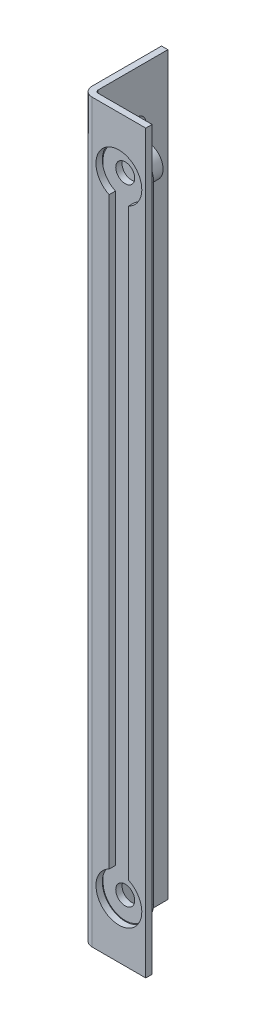
from build123d import *

# Parameters (mm, degrees)
BOSS_EXTRUDE1_DEPTH = 233
SKETCH2_R           = 3.15
CUT_EXTRUDE1_DEPTH  = 235.882949573
CUT_EXTRUDE2_DEPTH  = 235.985105911
SKETCH4_R           = 3
BOSS_EXTRUDE2_DEPTH = 2
SKETCH5_R           = 4.976227588
BOSS_EXTRUDE3_DEPTH = 5


with BuildPart() as part:
    # Sketch1 → Boss-Extrude1 (new body)
    with BuildSketch(Plane(origin=(0, 0, 0), x_dir=(1, 0, 0), z_dir=(0, 1, 0))):
        with BuildLine():
            Line((0, 0), (-17, 0))
            ThreePointArc((-17, 0), (-19.121320344, 0.878679656), (-20, 3))
            Line((-20, 3), (-20, 8.423888846))
            Line((-20, 8.423888846), (-20, 25))
            Line((-20, 25), (-18, 25))
            Line((-18, 25), (-18, 8.423888846))
            Line((-18, 8.423888846), (-18, 3))
            ThreePointArc((-18, 3), (-17.707106781, 2.292893219), (-17, 2))
            Line((-17, 2), (0, 2))
            Line((0, 2), (0, 0))
        make_face()
    extrude(amount=BOSS_EXTRUDE1_DEPTH)

    # Sketch2 → Cut-Extrude1 (cut, through all)
    with BuildSketch(Plane(origin=(-16, 0, 0), x_dir=(0, 0, -1), z_dir=(1, 0, 0))):
        with Locations((15, 116.173206962)):
            Circle(SKETCH2_R)
        with BuildLine():
            Line((18.1, 216.35), (18.1, 191.65))
            ThreePointArc((18.1, 191.65), (15, 188.55), (11.9, 191.65))
            Line((11.9, 191.65), (11.9, 216.35))
            ThreePointArc((11.9, 216.35), (15, 219.45), (18.1, 216.35))
        make_face()
        with BuildLine():
            Line((18.1, 41.35), (18.1, 16.65))
            ThreePointArc((18.1, 16.65), (15, 13.55), (11.9, 16.65))
            Line((11.9, 16.65), (11.9, 41.35))
            ThreePointArc((11.9, 41.35), (15, 44.45), (18.1, 41.35))
        make_face()
    extrude(amount=-CUT_EXTRUDE1_DEPTH, mode=Mode.SUBTRACT)

    # Sketch3 → Cut-Extrude2 (cut, through all)
    with BuildSketch(Plane(origin=(0, 0, -2), x_dir=(-1, 0, 0), z_dir=(0, 0, -1))):
        with BuildLine():
            Line((5.4, 208.946184318), (5.4, 24.053815682))
            ThreePointArc((5.4, 24.053815682), (8.5, 10.25), (11.6, 24.053815682))
            Line((11.6, 24.053815682), (11.6, 208.946184318))
            ThreePointArc((11.6, 208.946184318), (8.5, 222.75), (5.4, 208.946184318))
        make_face()
    extrude(amount=-CUT_EXTRUDE2_DEPTH, mode=Mode.SUBTRACT)

    # Sketch4 → Boss-Extrude2 (add)
    with BuildSketch(Plane(origin=(0, 0, -2), x_dir=(-1, 0, 0), z_dir=(0, 0, -1))):
        with BuildLine():
            Line((1.5, 215.5), (1.5, 17.5))
            ThreePointArc((1.5, 17.5), (8.5, 10.5), (15.5, 17.5))
            Line((15.5, 17.5), (15.5, 215.5))
            ThreePointArc((15.5, 215.5), (8.5, 222.5), (1.5, 215.5))
        make_face()
        with Locations((8.5, 215.5)):
            Circle(SKETCH4_R, mode=Mode.SUBTRACT)
        with Locations((8.5, 17.5)):
            Circle(SKETCH4_R, mode=Mode.SUBTRACT)
    extrude(amount=BOSS_EXTRUDE2_DEPTH)


with BuildPart() as body_2:
    # Sketch5 → Boss-Extrude3 (new body)
    with BuildSketch(Plane(origin=(0, 0, -4), x_dir=(-1, 0, 0), z_dir=(0, 0, -1))):
        with Locations((8.5, 215.5)):
            Circle(SKETCH5_R)
    extrude(amount=BOSS_EXTRUDE3_DEPTH)


solid = Compound([part.part, body_2.part])
